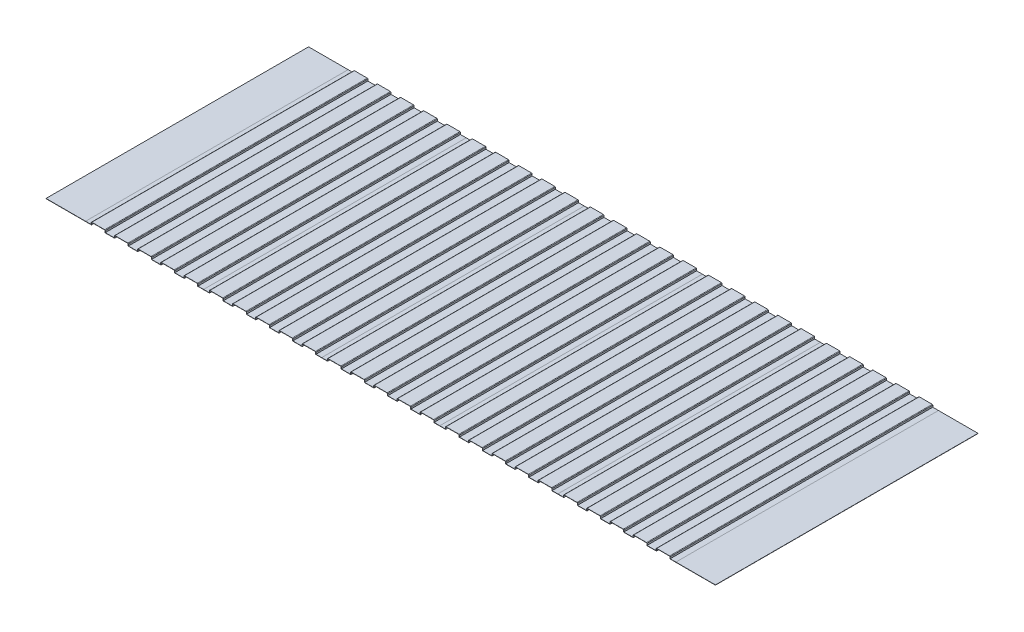
from build123d import *

# Parameters (mm, degrees)
BOSS_EXTRUDE1_DEPTH = 2324
LPATTERN1_COUNT     = 5
LPATTERN1_PITCH     = 1045
SKETCH2_W           = 2324
SKETCH2_H           = 2
BOSS_EXTRUDE2_DEPTH = 350
SKETCH3_W           = 2324
SKETCH3_H           = 2
BOSS_EXTRUDE3_DEPTH = 350


with BuildPart() as part:
    # Sketch1 → Boss-Extrude1 (new body)
    with BuildSketch(Plane.XY):
        with BuildLine():
            Line((1045, 2), (994.5, 2))
            Line((994.5, 2), (994.5, 17))
            ThreePointArc((994.5, 17), (993.035533906, 20.535533906), (989.5, 22))
            Line((989.5, 22), (875.5, 22))
            ThreePointArc((875.5, 22), (871.964466094, 20.535533906), (870.5, 17))
            Line((870.5, 17), (870.5, 2))
            Line((870.5, 2), (789.5, 2))
            Line((789.5, 2), (789.5, 17))
            ThreePointArc((789.5, 17), (788.035533906, 20.535533906), (784.5, 22))
            Line((784.5, 22), (670.5, 22))
            ThreePointArc((670.5, 22), (666.964466094, 20.535533906), (665.5, 17))
            Line((665.5, 17), (665.5, 2))
            Line((665.5, 2), (584.5, 2))
            Line((584.5, 2), (584.5, 17))
            ThreePointArc((584.5, 17), (583.035533906, 20.535533906), (579.5, 22))
            Line((579.5, 22), (465.5, 22))
            ThreePointArc((465.5, 22), (461.964466094, 20.535533906), (460.5, 17))
            Line((460.5, 17), (460.5, 2))
            Line((460.5, 2), (379.5, 2))
            Line((379.5, 2), (379.5, 17))
            ThreePointArc((379.5, 17), (378.035533906, 20.535533906), (374.5, 22))
            Line((374.5, 22), (260.5, 22))
            ThreePointArc((260.5, 22), (256.964466094, 20.535533906), (255.5, 17))
            Line((255.5, 17), (255.5, 2))
            Line((255.5, 2), (174.5, 2))
            Line((174.5, 2), (174.5, 17))
            ThreePointArc((174.5, 17), (173.035533906, 20.535533906), (169.5, 22))
            Line((169.5, 22), (55.5, 22))
            ThreePointArc((55.5, 22), (51.964466094, 20.535533906), (50.5, 17))
            Line((50.5, 17), (50.5, 2))
            Line((50.5, 2), (0, 2))
            Line((0, 2), (0, 0))
            Line((0, 0), (52.5, 0))
            Line((52.5, 0), (52.5, 17))
            ThreePointArc((52.5, 17), (53.378679656, 19.121320344), (55.5, 20))
            Line((55.5, 20), (169.5, 20))
            ThreePointArc((169.5, 20), (171.621320344, 19.121320344), (172.5, 17))
            Line((172.5, 17), (172.5, 0))
            Line((172.5, 0), (257.5, 0))
            Line((257.5, 0), (257.5, 17))
            ThreePointArc((257.5, 17), (258.378679656, 19.121320344), (260.5, 20))
            Line((260.5, 20), (374.5, 20))
            ThreePointArc((374.5, 20), (376.621320344, 19.121320344), (377.5, 17))
            Line((377.5, 17), (377.5, 0))
            Line((377.5, 0), (462.5, 0))
            Line((462.5, 0), (462.5, 17))
            ThreePointArc((462.5, 17), (463.378679656, 19.121320344), (465.5, 20))
            Line((465.5, 20), (579.5, 20))
            ThreePointArc((579.5, 20), (581.621320344, 19.121320344), (582.5, 17))
            Line((582.5, 17), (582.5, 0))
            Line((582.5, 0), (667.5, 0))
            Line((667.5, 0), (667.5, 17))
            ThreePointArc((667.5, 17), (668.378679656, 19.121320344), (670.5, 20))
            Line((670.5, 20), (784.5, 20))
            ThreePointArc((784.5, 20), (786.621320344, 19.121320344), (787.5, 17))
            Line((787.5, 17), (787.5, 0))
            Line((787.5, 0), (872.5, 0))
            Line((872.5, 0), (872.5, 17))
            ThreePointArc((872.5, 17), (873.378679656, 19.121320344), (875.5, 20))
            Line((875.5, 20), (989.5, 20))
            ThreePointArc((989.5, 20), (991.621320344, 19.121320344), (992.5, 17))
            Line((992.5, 17), (992.5, 0))
            Line((992.5, 0), (1045, 0))
            Line((1045, 0), (1045, 2))
        make_face()
    extrude(amount=BOSS_EXTRUDE1_DEPTH)


with BuildPart() as lpattern1_1:
    # LPattern1: pattern copy
    add(part.part.moved(Location(Vector(1, 0, 0) * (1 * LPATTERN1_PITCH))))


with BuildPart() as lpattern1_2:
    # LPattern1: pattern copy
    add(part.part.moved(Location(Vector(1, 0, 0) * (2 * LPATTERN1_PITCH))))


with BuildPart() as lpattern1_3:
    # LPattern1: pattern copy
    add(part.part.moved(Location(Vector(1, 0, 0) * (3 * LPATTERN1_PITCH))))


with BuildPart() as lpattern1_4:
    # LPattern1: pattern copy
    add(part.part.moved(Location(Vector(1, 0, 0) * (4 * LPATTERN1_PITCH))))


with BuildPart() as body_6:
    # Sketch2 → Boss-Extrude2 (new body)
    with BuildSketch(Plane.ZY):
        with Locations((1162, 1)):
            Rectangle(SKETCH2_W, SKETCH2_H)
    extrude(amount=BOSS_EXTRUDE2_DEPTH)


with BuildPart() as body_7:
    # Sketch3 → Boss-Extrude3 (new body)
    with BuildSketch(Plane(origin=(5225, 0, 0), x_dir=(0, 0, -1), z_dir=(1, 0, 0))):
        with Locations((-1162, 1)):
            Rectangle(SKETCH3_W, SKETCH3_H)
    extrude(amount=BOSS_EXTRUDE3_DEPTH)


solid = Compound([part.part, lpattern1_1.part, lpattern1_2.part, lpattern1_3.part, lpattern1_4.part, body_6.part, body_7.part])
